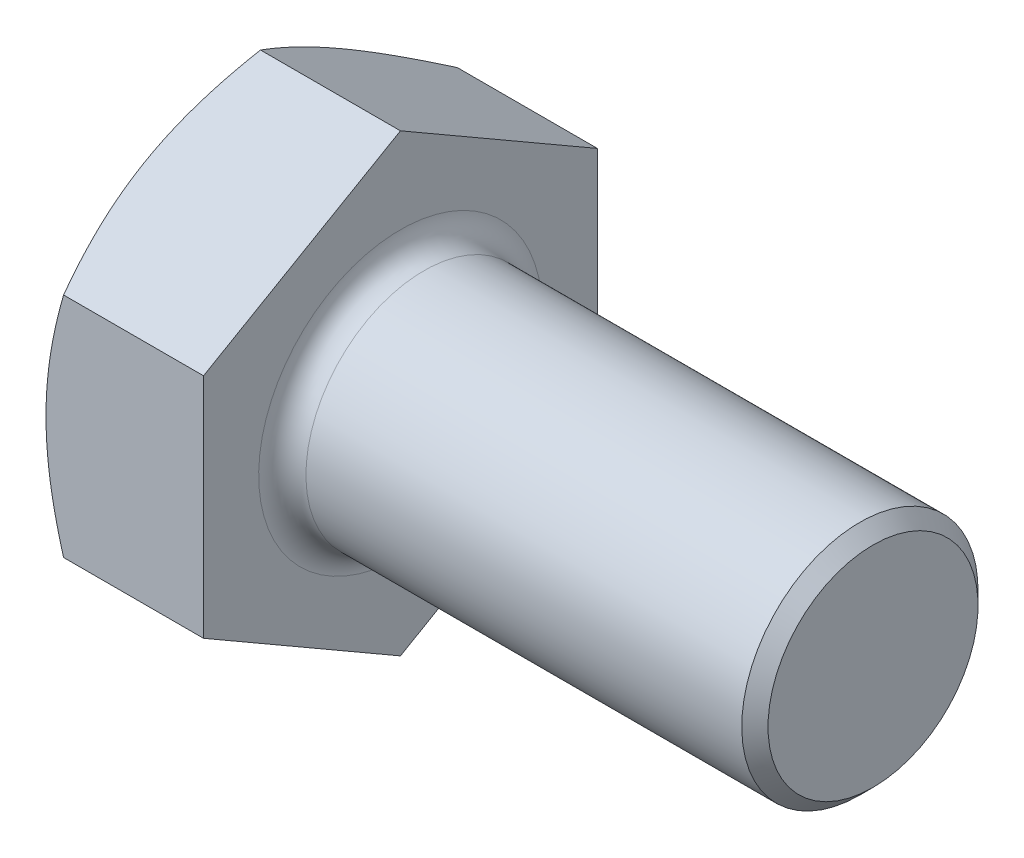
from build123d import *

# Parameters (mm, degrees)
EXTRUDE_1_DEPTH     = 4
SKETCH_4_R          = 10.89
SKETCH_4_R_2        = 5
CUT_EXTRUDE_1_DEPTH = 0.5
CUT_EXTRUDE_1_DRAFT = -60
CHAMFER_2_SIZE      = 0.333333333


with BuildPart() as part:
    # 草图3 → 凸台-拉伸1 (new body)
    with BuildSketch(Plane(origin=(0, 0, 0), x_dir=(0, 0, -1), z_dir=(1, 0, 0))):
        Polygon((5, 2.886751346), (0, 5.773502692), (-5, 2.886751346), (-5, -2.886751346), (0, -5.773502692), (5, -2.886751346), align=None)
    extrude(amount=EXTRUDE_1_DEPTH)


with BuildPart() as cut_extrude_1_tool:
    # 草图4 → 切除-拉伸1 (with draft: the straight prism first)
    with BuildSketch(Plane.ZY):
        Circle(SKETCH_4_R)
        Circle(SKETCH_4_R_2, mode=Mode.SUBTRACT)
    extrude(amount=-CUT_EXTRUDE_1_DEPTH)
    # 切除-拉伸1: the draft: its side faces are tilted about the plane it starts from
    cut_extrude_1_sides = [cut_extrude_1_tool.faces().sort_by_distance(p)[0] for p in [
        (0.25, 0, -10.89),
        (0.25, 0, -5),
    ]]
    draft(cut_extrude_1_sides, Plane.ZY, CUT_EXTRUDE_1_DRAFT)


with BuildPart() as part_1:
    add(part.part)

    # 切除-拉伸1: cut by cut_extrude_1_tool
    add(cut_extrude_1_tool.part, mode=Mode.SUBTRACT)

    # 草图5 → 旋转1 (revolve)
    with BuildSketch(Plane.XY, mode=Mode.PRIVATE) as revolve_1_sk:
        with BuildLine():
            Line((4.6, 3), (16, 3))
            Line((16, 3), (16, 0))
            Line((16, 0), (4, 0))
            Line((4, 0), (4, 3.6))
            ThreePointArc((4, 3.6), (4.175735931, 3.175735931), (4.6, 3))
        make_face()
    revolve(revolve_1_sk.sketch.rotate(Axis((4, 0, 0), (1, 0, 0)), 180), axis=Axis((4, 0, 0), (1, 0, 0)))

    # 倒角2
    chamfer_2_edges = [part_1.edges().sort_by_distance(p)[0] for p in [
        (16, 3, 0),
    ]]
    chamfer(chamfer_2_edges, length=CHAMFER_2_SIZE)


solid = part_1.part
